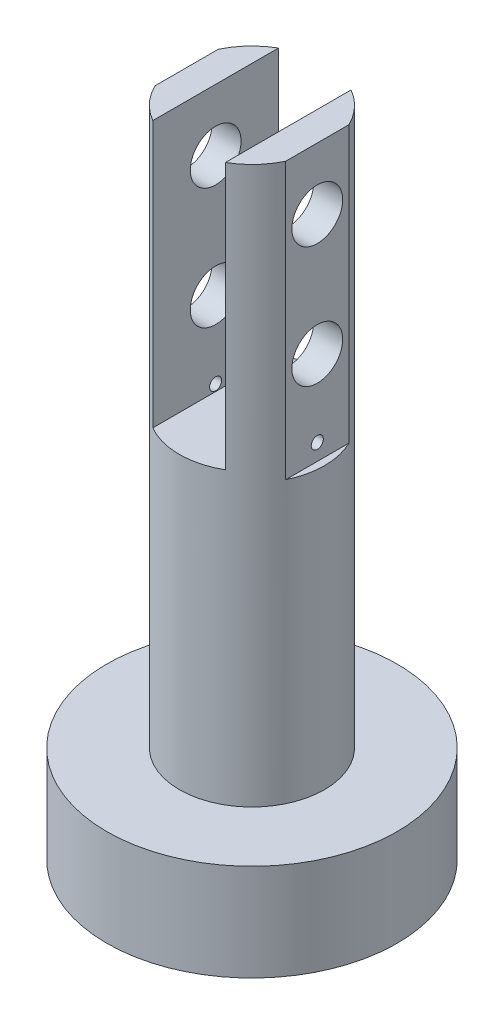
SolidWorks part; units mm, degrees
ref_plane "前视基准面" through (0, 0, 0) normal (0, 0, 1) x (1, 0, 0)
ref_plane "上视基准面" through (0, 0, 0) normal (0, 1, 0) x (1, 0, 0)
ref_plane "右视基准面" through (0, 0, 0) normal (1, 0, 0) x (0, 0, -1)
sketch "草图1" plane through (0, 0, 0) normal (0, 1, 0) x (1, 0, 0)
  circle A0 centre (0, 0) radius 30
  dimension "D1" = 60
extrude "凸台-拉伸1" add sketch "草图1" along normal blind 20
sketch "草图2" plane through (0, 20, 0) normal (0, 1, 0) x (1, 0, 0)
  circle A0 centre (0, 0) radius 15
  dimension "D1" = 30
extrude "凸台-拉伸2" add sketch "草图2" along normal blind 115
sketch "草图3" plane through (0, 0, 0) normal (0, 0, 1) x (1, 0, 0)
  line L1 (-7.5, 80) -> (7.5, 80)
  line L2 (-7.5, 80) -> (-7.5, 145.2752)
  line L3 (-7.5, 145.2752) -> (7.5, 145.2752)
  line L4 (7.5, 80) -> (7.5, 145.2752)
  line L5 (15, 135) -> (-15, 135) construction
  point P4 (0, 80)
  dimension "D1" = 15
  dimension "D2" = 55
extrude "切除-拉伸1" cut sketch "草图3" against normal mid plane 100
sketch "草图4" plane through (0, 0, 0) normal (0, 0, 1) x (1, 0, 0)
  line L0 (7.5, 135) -> (7.5, 80) construction
  line L1 (24.7145, 78) -> (13.5, 78)
  line L2 (24.7145, 78) -> (24.7145, 151.1462)
  line L3 (24.7145, 151.1462) -> (13.5, 151.1462)
  line L4 (13.5, 78) -> (13.5, 151.1462)
  line L5 (-24.7145, 78) -> (-13.5, 78)
  line L6 (-24.7145, 78) -> (-24.7145, 151.1462)
  line L7 (-24.7145, 151.1462) -> (-13.5, 151.1462)
  line L8 (-13.5, 78) -> (-13.5, 151.1462)
  line L9 (-7.5, 80) -> (-7.5, 135) construction
  line L10 (-7.5, 135) -> (-15, 135) construction
  point P14 (-19.1073, 78)
  dimension "D1" = 6
  dimension "D2" = 6
  dimension "D3" = 57
extrude "切除-拉伸2" cut sketch "草图4" against normal mid plane 50
hole_wizard "Ø10.5 (10.5) 直径孔1" positions "草图5" profile "草图6" hole size "Ø10.5" standard "GB" end condition through all
sketch "草图5" plane through (13.5, 0, 0) normal (1, 0, 0) x (0, 0, -1)
  line L0 (6.5383, 135) -> (-6.5383, 135) construction
  point P0 (0, 97.25)
  point P2 (0, 122.25)
  point P10 (0, 135)
  dimension "D1" = 12.75
  dimension "D2" = 25
sketch "草图6" plane through (13.5, 97.25, 0) normal (0, 1, 0) x (0, 0, -1)
  line L0 (0, 0) -> (0, 43.5)
  line L1 (0, 43.5) -> (5.25, 43.5)
  line L2 (5.25, 43.5) -> (5.25, 0)
  line L5 (5.25, 0) -> (0, 0)
  line L11 (0, -6.35) -> (0, 107.95) construction
  dimension "通孔孔直径" = 10.5
  dimension "通孔孔深度" = 43.5
hole_wizard "M3 螺纹孔1" positions "草图7" profile "草图8" tap size "M3" standard "GB" end condition through all
sketch "草图7" plane through (-13.5, 0, 0) normal (-1, 0, 0) x (0, 0, 1)
  line L0 (6.5383, 135) -> (-6.5383, 135) construction
  line L1 (6.5383, 78) -> (-6.5383, 78) construction
  point P0 (0, 81.4)
  point P5 (0, 135)
  dimension "D1" = 3.4
sketch "草图8" plane through (-13.5, 81.4, 0) normal (0, 1, 0) x (0, 0, 1)
  line L0 (0, 0) -> (0, 43.5)
  line L1 (0, 43.5) -> (1.25, 43.5)
  line L2 (1.25, 43.5) -> (1.25, 0)
  line L5 (1.25, 0) -> (0, 0)
  line L11 (0, -6.35) -> (0, 107.95) construction
  dimension "通孔螺纹孔钻头直径" = 2.5
  dimension "通孔螺纹孔钻头深度" = 43.5
cosmetic thread "孔螺蚊线1" parameters "D2"=3
